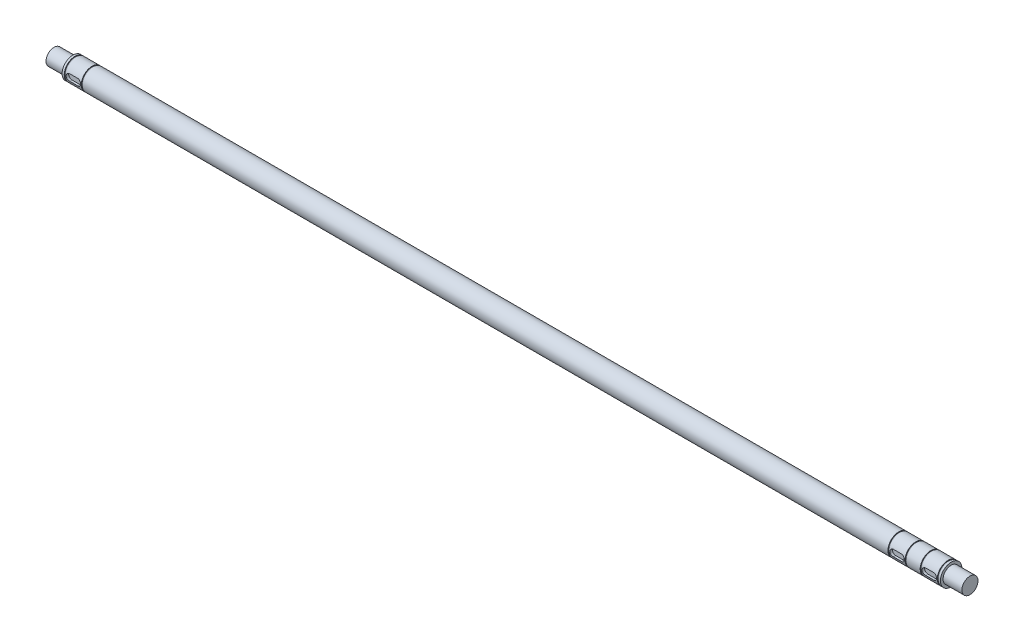
SolidWorks part; units mm, degrees
ref_plane "前视基准面" through (0, 0, 0) normal (0, 0, 1) x (1, 0, 0)
ref_plane "上视基准面" through (0, 0, 0) normal (0, 1, 0) x (1, 0, 0)
ref_plane "右视基准面" through (0, 0, 0) normal (1, 0, 0) x (0, 0, -1)
sketch "草图1" plane through (0, 0, 0) normal (1, 0, 0) x (0, 0, -1)
  circle A0 centre (0, 0) radius 20
  dimension "D1" = 40
extrude "凸台-拉伸1" add sketch "草图1" along normal blind 1635.36
sketch "草图2" plane through (0, 0, 0) normal (-1, 0, 0) x (0, 0, 1)
  circle A0 centre (0, 0) radius 15
  dimension "D1" = 30
extrude "凸台-拉伸2" add sketch "草图2" along normal blind 35
sketch "草图3" plane through (1635.36, 0, 0) normal (1, 0, 0) x (0, 0, -1)
  circle A0 centre (0, 0) radius 15
  dimension "D1" = 30
extrude "凸台-拉伸3" add sketch "草图3" along normal blind 35
ref_plane "基准面1" through (0, 0, 15) normal (0, 0, 1) x (1, 0, 0)
sketch "草图4" plane through (0, 0, 15) normal (0, 0, 1) x (1, 0, 0)
  line L0 (13.3, 0) -> (28.3, 0) construction
  line L1 (13.3, 6) -> (28.3, 6)
  line L2 (13.3, -6) -> (28.3, -6)
  line L3 (1622.06, 0) -> (1607.06, 0) construction
  line L4 (1622.06, -6) -> (1607.06, -6)
  line L5 (1622.06, 6) -> (1607.06, 6)
  line L6 (0, 0) -> (1810.9625, 0) construction
  line L7 (0, 20) -> (0, -20) construction
  line L8 (1635.36, -20) -> (1635.36, 20) construction
  line L9 (-60, 0) -> (1750.9625, 0) construction
  line L10 (1562.06, 0) -> (1547.06, 0) construction
  line L11 (1562.06, -6) -> (1547.06, -6)
  line L12 (1562.06, 6) -> (1547.06, 6)
  arc A0 (13.3, 6) -> (13.3, -6) centre (13.3, 0) ccw
  arc A1 (28.3, -6) -> (28.3, 6) centre (28.3, 0) ccw
  arc A2 (1622.06, -6) -> (1622.06, 6) centre (1622.06, 0) ccw
  arc A3 (1607.06, 6) -> (1607.06, -6) centre (1607.06, 0) ccw
  arc A4 (1562.06, -6) -> (1562.06, 6) centre (1562.06, 0) ccw
  arc A5 (1547.06, 6) -> (1547.06, -6) centre (1547.06, 0) ccw
  point P3 (20.8, 0)
  point P8 (1614.56, 0)
  point P23 (1554.56, 0)
  dimension "D1" = 12
  dimension "D2" = 12
  dimension "D3" = 15
  dimension "D4" = 15
  dimension "D5" = 20.8
  dimension "D6" = 20.8
  dimension "D8" = 60
  dimension "D7" = 2
extrude "切除-拉伸1" cut sketch "草图4" along normal through all
sketch "草图5" plane through (0, 0, 0) normal (0, 0, 1) x (1, 0, 0)
  line L0 (1635.36, 20) -> (0, 20) construction
  line L1 (3.95, 20) -> (5.8, 20)
  line L2 (3.95, 20) -> (3.95, 18.75)
  line L3 (3.95, 18.75) -> (5.8, 18.75)
  line L4 (5.8, 20) -> (5.8, 18.75)
  line L5 (20.8, -6) -> (20.8, 38.1679) construction
  line L6 (35.8, 20) -> (37.65, 20)
  line L7 (35.8, 20) -> (35.8, 18.75)
  line L8 (35.8, 18.75) -> (37.65, 18.75)
  line L9 (37.65, 20) -> (37.65, 18.75)
  line L10 (13.3, -6) -> (28.3, -6) construction
  line L11 (0, 0) -> (42.6783, 0) construction
  dimension "D1" = 1.85
  dimension "D2" = 18.75
  dimension "D3" = 30
revolve "切除-旋转1" cut sketch "草图5" angle 360 about L11
sketch "草图7" plane through (0, 0, 0) normal (0, 0, 1) x (1, 0, 0)
  line L0 (1614.56, -6) -> (1614.56, 18.7729) construction
  line L1 (1607.06, -6) -> (1622.06, -6) construction
  line L2 (1635.36, 20) -> (37.65, 20) construction
  line L3 (1597.71, 20) -> (1599.56, 20)
  line L4 (1597.71, 20) -> (1597.71, 18.75)
  line L5 (1597.71, 18.75) -> (1599.56, 18.75)
  line L6 (1599.56, 20) -> (1599.56, 18.75)
  line L7 (1670.36, 0) -> (1562.06, 0) construction
  line L8 (1629.56, 20) -> (1631.41, 20)
  line L9 (1629.56, 20) -> (1629.56, 18.75)
  line L10 (1629.56, 18.75) -> (1631.41, 18.75)
  line L11 (1631.41, 20) -> (1631.41, 18.75)
  line L12 (1670.36, -15) -> (1670.36, 15) construction
  dimension "D1" = 1.85
  dimension "D2" = 18.75
  dimension "D3" = 30
revolve "切除-旋转2" cut sketch "草图7" angle 360 about L7
pattern_linear "阵列(线性)2" count 2 spacing 60 along (-1, 0, 0) of "切除-旋转2"
